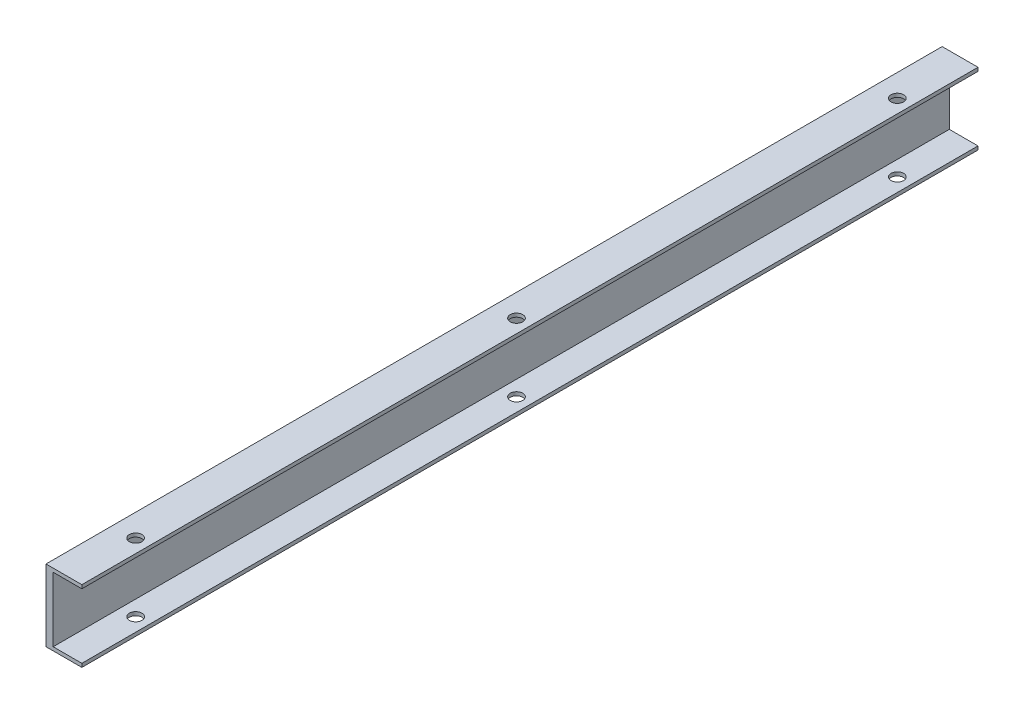
from build123d import *

# Parameters (mm, degrees)
EXTRUDE1_DEPTH     = 1000
SKETCH2_R          = 7
CUT_EXTRUDE1_DEPTH = 1004.992031841
LPATTERN1_COUNT    = 3
LPATTERN1_PITCH    = 425


with BuildPart() as part:
    # Sketch1 → Extrude1 (new body)
    with BuildSketch(Plane.XY):
        Polygon((0, 0), (-40, 0), (-40, 80), (0, 80), (0, 76), (-32, 76), (-32, 4), (0, 4), align=None)
    extrude(amount=EXTRUDE1_DEPTH)

    # Sketch2 → Cut-Extrude1 (cut, through all)
    with BuildSketch(Plane(origin=(0, 80, 0), x_dir=(1, 0, 0), z_dir=(0, 1, 0))):
        with Locations(Location((-15, -925, 0), (0, 0, 270))):
            Circle(SKETCH2_R)
    cut_extrude1 = extrude(amount=-CUT_EXTRUDE1_DEPTH, mode=Mode.SUBTRACT)

    # LPattern1: Cut-Extrude1 ×3
    with Locations(*[(0, 0, -i * LPATTERN1_PITCH) for i in range(1, LPATTERN1_COUNT)]):
        add(cut_extrude1, mode=Mode.SUBTRACT)


solid = part.part
